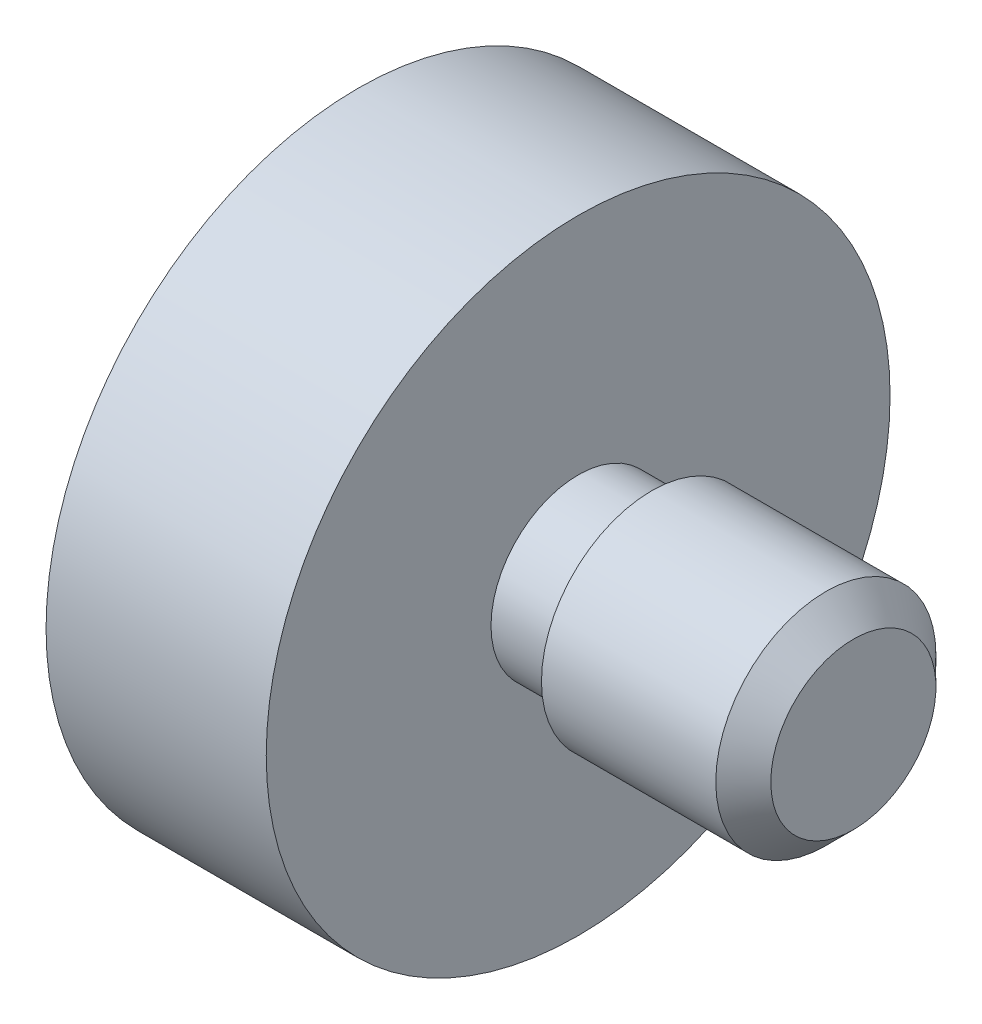
from build123d import *

# Parameters (mm, degrees)
CHAMFER1_SIZE = 1.5


with BuildPart() as part:
    # Sketch1 → Revolve1 (revolve)
    with BuildSketch(Plane.XY, mode=Mode.PRIVATE) as revolve1_sk:
        Polygon((0, 0), (0, 17), (12, 17), (12, 4.75), (16, 4.75), (16, 6), (27, 6), (27, 0), align=None)
    revolve(revolve1_sk.sketch.rotate(Axis((0, 0, 0), (1, 0, 0)), 90), axis=Axis((0, 0, 0), (1, 0, 0)))

    # Chamfer1
    chamfer1_edges = [part.edges().sort_by_distance(p)[0] for p in [
        (27, 0, -6),
    ]]
    chamfer(chamfer1_edges, length=CHAMFER1_SIZE)

    # Sketch2 → Cut-Revolve1 (revolve, cut)
    with BuildSketch(Plane.XY, mode=Mode.PRIVATE) as cut_revolve1_sk:
        Polygon((0, 11), (0, 13), (6, 13), (7.154700538, 11), align=None)
    cut_revolve1 = revolve(cut_revolve1_sk.sketch.rotate(Axis((-2.466856423, 11, 0), (1, 0, 0)), 90), axis=Axis((-2.466856423, 11, 0), (1, 0, 0)), mode=Mode.SUBTRACT)

    # Mirror1: Cut-Revolve1 across plane
    add(cut_revolve1.mirror(Plane.ZX), mode=Mode.SUBTRACT)


solid = part.part
